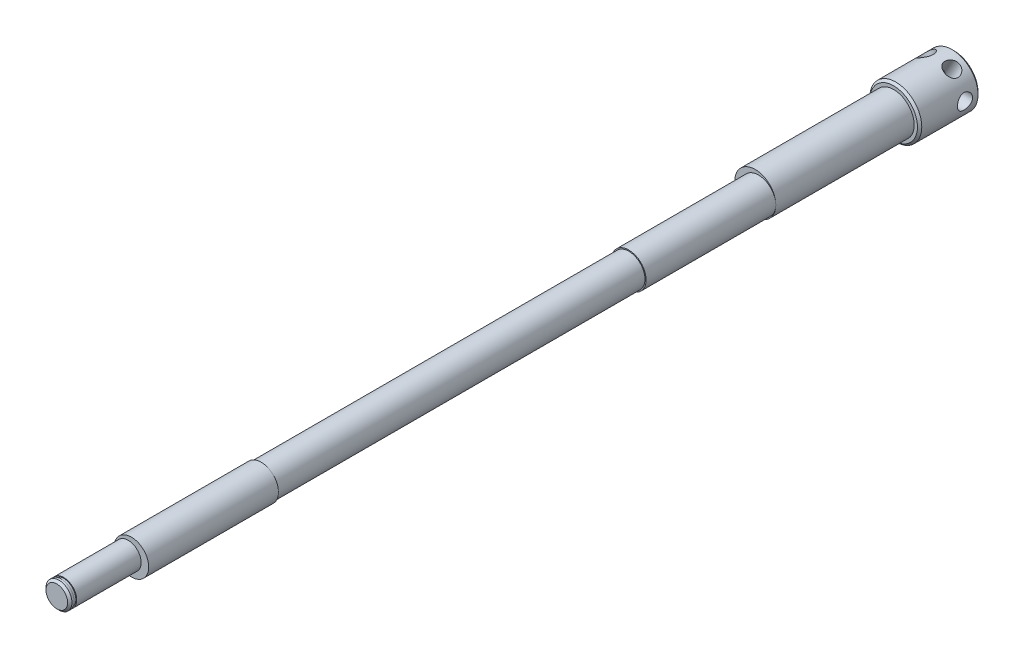
from build123d import *

# Parameters (mm, degrees)
SKETCH1_R           = 6
BOSS_EXTRUDE1_DEPTH = 7
SKETCH2_R           = 4.75
BOSS_EXTRUDE2_DEPTH = 32
SKETCH3_R           = 4
BOSS_EXTRUDE3_DEPTH = 30
SKETCH4_R           = 3.75
BOSS_EXTRUDE4_DEPTH = 85
SKETCH5_R           = 4
BOSS_EXTRUDE5_DEPTH = 30
SKETCH6_R           = 3
BOSS_EXTRUDE6_DEPTH = 16.5
SKETCH8_W           = 1.531468115
SKETCH8_H           = 0.6
CHAMFER1_SIZE       = 0.5
SKETCH11_R          = 1.75
CUT_EXTRUDE1_DEPTH  = 11.5
CIRPATTERN1_COUNT   = 3
CIRPATTERN1_ANGLE   = 120
CHAMFER2_SIZE       = 0.5


with BuildPart() as part:
    # Sketch1 → Boss-Extrude1 (new, symmetric)
    with BuildSketch(Plane.XY):
        Circle(SKETCH1_R)
    extrude(amount=BOSS_EXTRUDE1_DEPTH, both=True)

    # Sketch2 → Boss-Extrude2 (add)
    with BuildSketch(Plane.XY.offset(7)):
        Circle(SKETCH2_R)
    extrude(amount=BOSS_EXTRUDE2_DEPTH)

    # Sketch3 → Boss-Extrude3 (add)
    with BuildSketch(Plane.XY.offset(39)):
        with Locations((0.75, 0)):
            Circle(SKETCH3_R)
    extrude(amount=BOSS_EXTRUDE3_DEPTH)

    # Sketch4 → Boss-Extrude4 (add)
    with BuildSketch(Plane.XY.offset(69)):
        with Locations((0.75, 0)):
            Circle(SKETCH4_R)
    extrude(amount=BOSS_EXTRUDE4_DEPTH)

    # Sketch5 → Boss-Extrude5 (add)
    with BuildSketch(Plane.XY.offset(154)):
        with Locations((0.75, 0)):
            Circle(SKETCH5_R)
    extrude(amount=BOSS_EXTRUDE5_DEPTH)

    # Sketch6 → Boss-Extrude6 (add)
    with BuildSketch(Plane.XY.offset(184)):
        Circle(SKETCH6_R)
    extrude(amount=BOSS_EXTRUDE6_DEPTH)

    # Sketch8 → Cut-Revolve1 (revolve, cut)
    with BuildSketch(Plane(origin=(0, 0, 0), x_dir=(1, 0, 0), z_dir=(0, 1, 0)), mode=Mode.PRIVATE) as cut_revolve1_sk:
        with Locations((3.565734058, -199.2)):
            Rectangle(SKETCH8_W, SKETCH8_H)
    revolve(cut_revolve1_sk.sketch.rotate(Axis((0, 0, 0), (0, 0, 1)), 180), axis=Axis((0, 0, 0), (0, 0, 1)), mode=Mode.SUBTRACT)

    # Chamfer1
    chamfer1_edges = [part.edges().sort_by_distance(p)[0] for p in [
        (-6, 0, -7),
        (-6, 0, 7),
    ]]
    chamfer(chamfer1_edges, length=CHAMFER1_SIZE)

    # Sketch11 → Cut-Extrude1 (cut, symmetric)
    with BuildSketch(Plane(origin=(0, 0, 0), x_dir=(0, 0, -1), z_dir=(1, 0, 0))):
        with Locations(Location((3.5, 0, 0), (0, 0, 180))):
            Circle(SKETCH11_R)
    cut_extrude1 = extrude(amount=CUT_EXTRUDE1_DEPTH, both=True, mode=Mode.SUBTRACT)

    # CirPattern1: Cut-Extrude1 ×3 about axis
    cirpattern1_axis = Axis((0, 0, 7), (0, 0, -1))
    for i in range(1, CIRPATTERN1_COUNT):
        add(cut_extrude1.rotate(cirpattern1_axis, i * CIRPATTERN1_ANGLE / (CIRPATTERN1_COUNT - 1)), mode=Mode.SUBTRACT)

    # Chamfer2
    chamfer2_edges = [part.edges().sort_by_distance(p)[0] for p in [
        (-3, 0, 200.5),
    ]]
    chamfer(chamfer2_edges, length=CHAMFER2_SIZE)


solid = part.part
